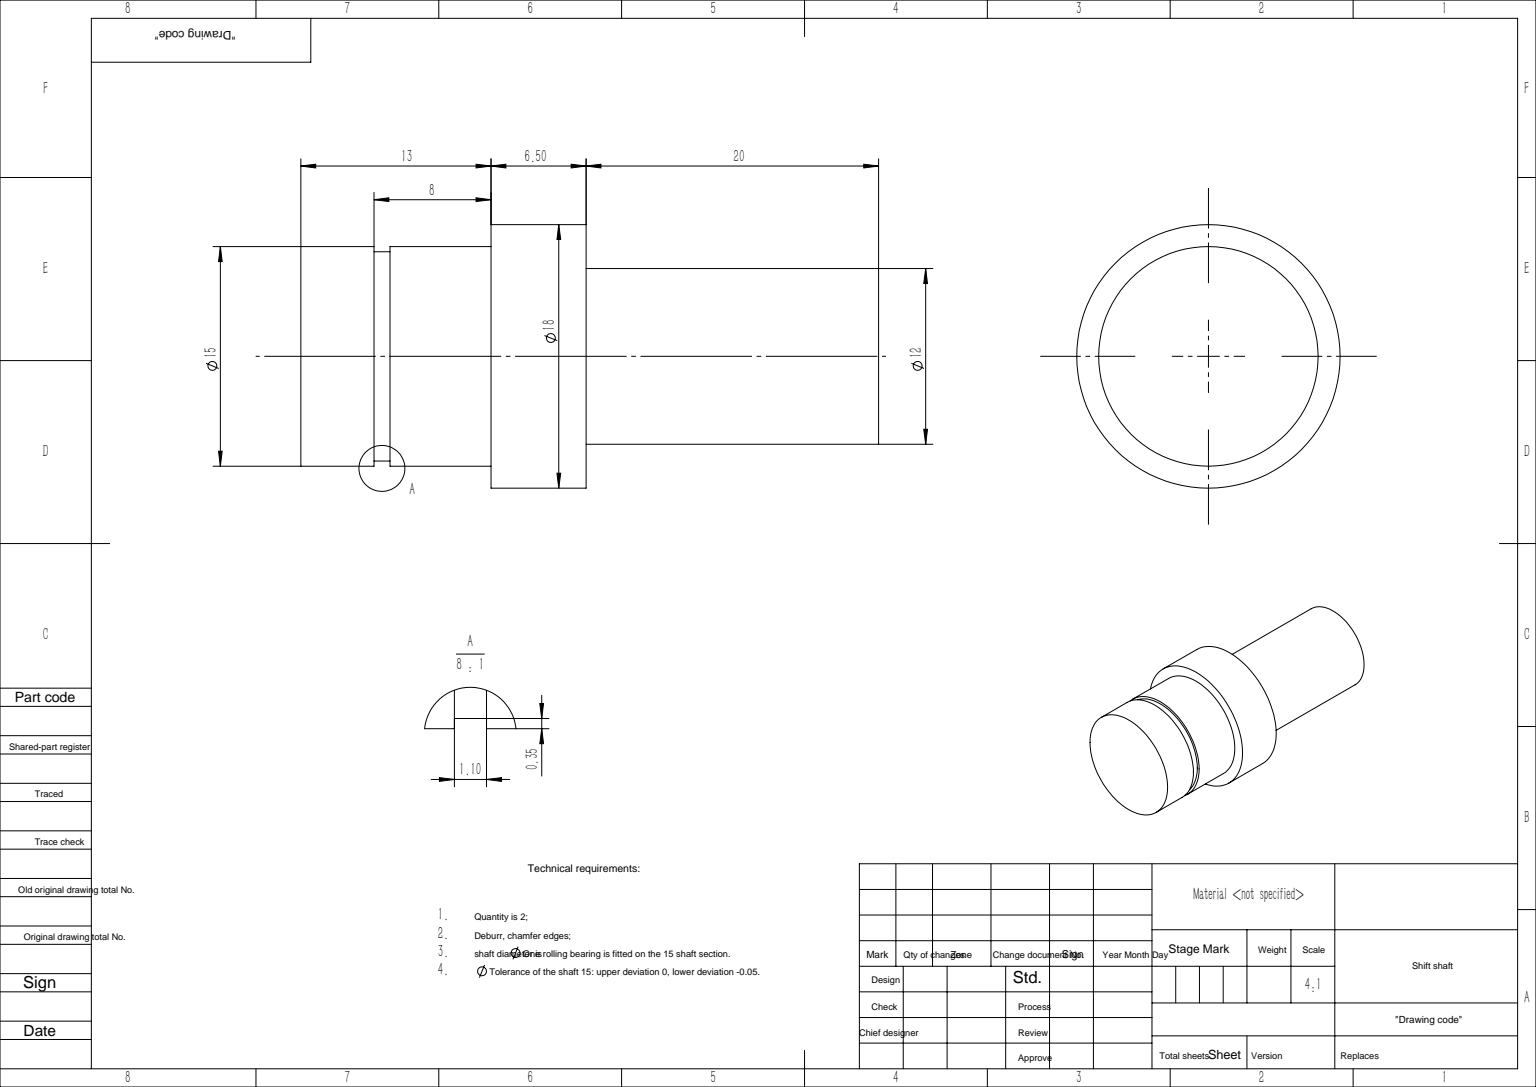
SolidWorks part; units mm, degrees
ref_plane "前视基准面" through (0, 0, 0) normal (0, 0, 1) x (1, 0, 0)
ref_plane "上视基准面" through (0, 0, 0) normal (0, 1, 0) x (1, 0, 0)
ref_plane "右视基准面" through (0, 0, 0) normal (1, 0, 0) x (0, 0, -1)
sketch "草图2" plane through (0, 0, 0) normal (1, 0, 0) x (0, 0, -1)
  line L0 (0, 0) -> (0, 7.5)
  line L1 (0, 7.5) -> (13, 7.5)
  line L2 (13, 7.5) -> (13, 9)
  line L3 (13, 9) -> (19.5, 9)
  line L4 (19.5, 9) -> (19.5, 6)
  line L5 (19.5, 6) -> (39.5, 6)
  line L6 (39.5, 6) -> (39.5, 0)
  line L7 (39.5, 0) -> (0, 0)
  dimension "D1" = 6
  dimension "D2" = 20
  dimension "D3" = 6.5
  dimension "D4" = 13
  dimension "D5" = 7.5
  dimension "D6" = 9
revolve "旋转1" add sketch "草图2" angle 360 about L7
ref_plane "基准面1" through (0, 0, -5) normal (0, 0, 1) x (1, 0, 0)
sketch "草图3" plane through (0, 0, -5) normal (0, 0, 1) x (1, 0, 0)
  circle A0 centre (0, 0) radius 7.5
  circle A1 centre (0, 0) radius 7.15
  circle A2 centre (0, 0) radius 7.5 construction
  dimension "D1" = 14.3
extrude "切除-拉伸1" cut sketch "草图3" against normal blind 1.1
